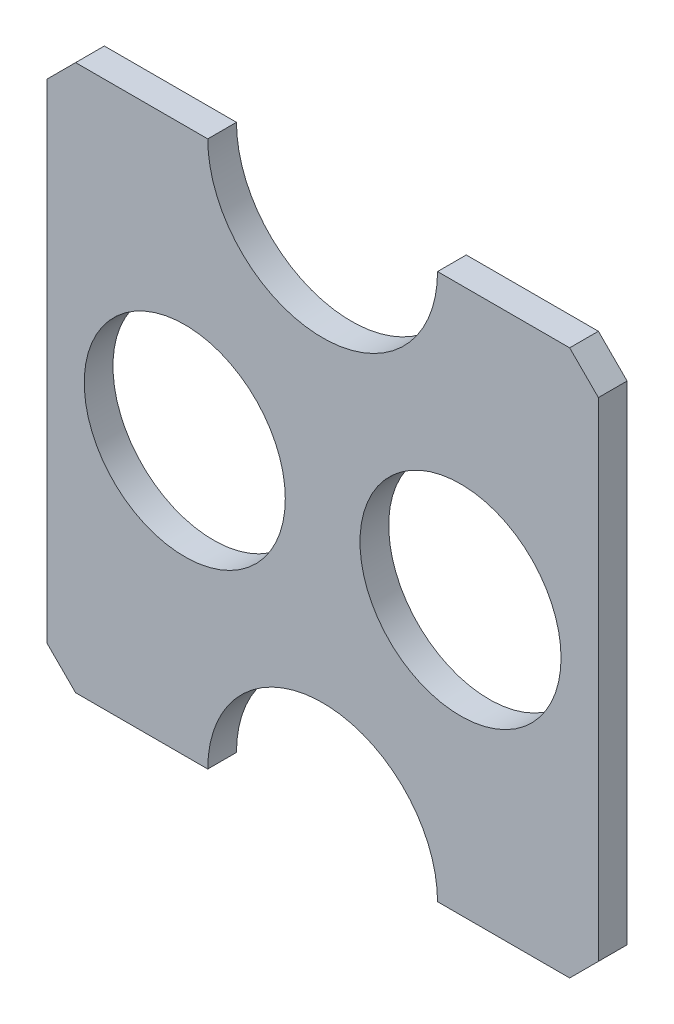
from build123d import *

# Parameters (mm, degrees)
SKETCH1_R           = 35
BOSS_EXTRUDE1_DEPTH = 10


with BuildPart() as part:
    # Sketch1 → Boss-Extrude1 (new body)
    with BuildSketch(Plane.XY):
        with BuildLine():
            Line((10, 0), (56, 0))
            ThreePointArc((56, 0), (96, 40), (136, 0))
            Line((136, 0), (182, 0))
            Line((182, 0), (192, 10))
            Line((192, 10), (192, 180))
            Line((192, 180), (182, 190))
            Line((182, 190), (136, 190))
            ThreePointArc((136, 190), (96, 150), (56, 190))
            Line((56, 190), (10, 190))
            Line((10, 190), (0, 180))
            Line((0, 180), (0, 10))
            Line((0, 10), (10, 0))
        make_face()
        with Locations((48, 95)):
            Circle(SKETCH1_R, mode=Mode.SUBTRACT)
        with Locations((144, 95)):
            Circle(SKETCH1_R, mode=Mode.SUBTRACT)
    extrude(amount=BOSS_EXTRUDE1_DEPTH)


solid = part.part
